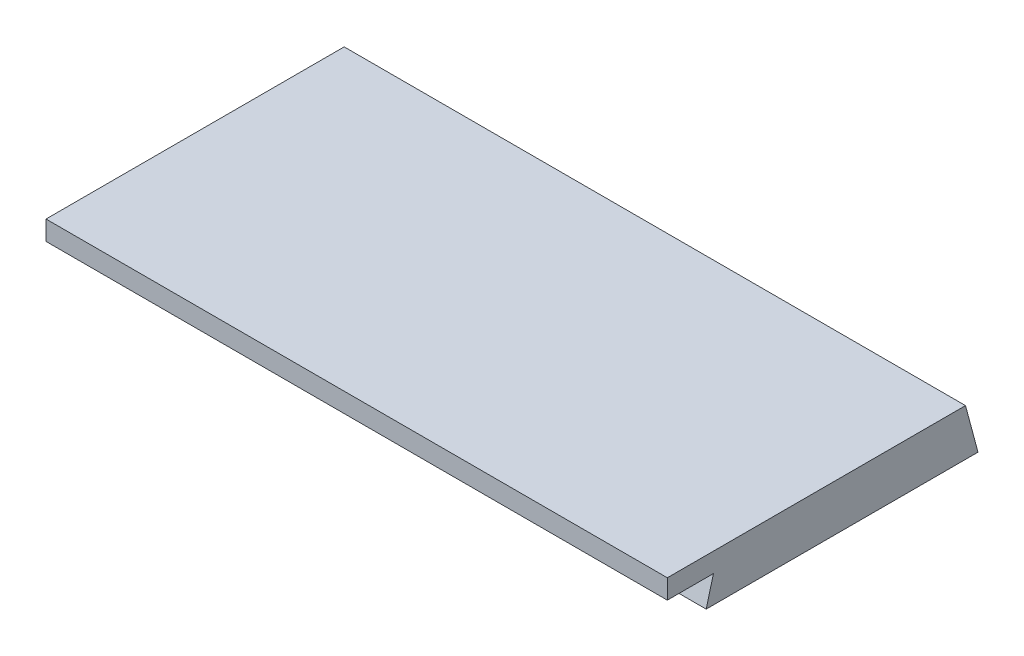
SolidWorks part; units mm, degrees
material "Q235-A"
ref_plane "Front Plane" through (0, 0, 0) normal (0, 0, 1) x (1, 0, 0)
ref_plane "Top Plane" through (0, 0, 0) normal (0, 1, 0) x (1, 0, 0)
ref_plane "Right Plane" through (0, 0, 0) normal (1, 0, 0) x (0, 0, -1)
sketch "Sketch1" plane through (0, 0, 0) normal (1, 0, 0) x (0, 0, -1)
  line L1 (350, 0) -> (333.923, 60)
  line L2 (333.923, 60) -> (-50, 60)
  line L3 (-50, 60) -> (-50, 35)
  line L4 (-50, 35) -> (9.3782, 35)
  line L5 (9.3782, 35) -> (0, 0)
  line L6 (0, 0) -> (350, 0)
  dimension "D1" = 400
  dimension "D2" = 60
  dimension "D3" = 75
  dimension "D4" = 25
  dimension "D5" = 75
  dimension "D6" = 350
extrude "Boss-Extrude1" add sketch "Sketch1" along normal mid plane 800
